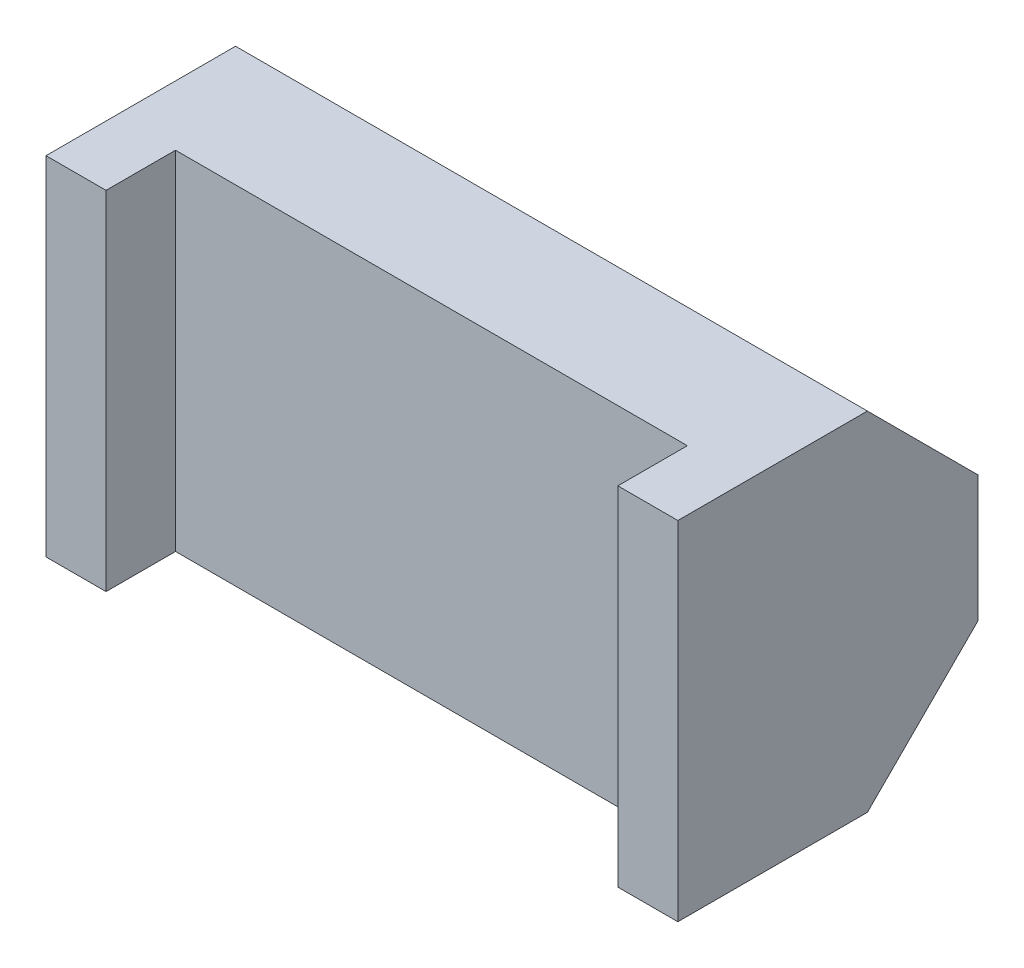
SolidWorks part; units mm, degrees
ref_plane "前视基准面" through (0, 0, 0) normal (0, 0, 1) x (1, 0, 0)
ref_plane "上视基准面" through (0, 0, 0) normal (0, 1, 0) x (1, 0, 0)
ref_plane "右视基准面" through (0, 0, 0) normal (1, 0, 0) x (0, 0, -1)
sketch "草图1" plane through (0, 0, 0) normal (0, 0, 1) x (1, 0, 0)
  line L0 (0, 5.5) -> (0, 0) construction
  line L1 (-10, 5.5) -> (10, 5.5)
  line L2 (-10, 5.5) -> (-10, -5.5)
  line L3 (-10, -5.5) -> (10, -5.5)
  line L4 (10, 5.5) -> (10, -5.5)
  line L5 (0, 0) -> (10, 0) construction
  dimension "D1" = 20
  dimension "D2" = 11
extrude "凸台-拉伸1" add sketch "草图1" along normal blind 9.5
sketch "草图2" plane through (0, 0, 9.5) normal (0, 0, 1) x (1, 0, 0)
  line L0 (0, 4.3603) -> (0, 0) construction
  line L1 (-8.1, 14.9476) -> (8.1, 14.9476)
  line L2 (-8.1, 14.9476) -> (-8.1, -14.9476)
  line L3 (-8.1, -14.9476) -> (8.1, -14.9476)
  line L4 (8.1, 14.9476) -> (8.1, -14.9476)
  line L5 (0, 0) -> (16.2, 0) construction
  dimension "D1" = 16.2
extrude "切除-拉伸1" cut sketch "草图2" against normal blind 2.2
sketch "草图3" plane through (-10, 0, 0) normal (-1, 0, 0) x (0, 0, 1)
  line L0 (0, 5.5) -> (3.5, 5.5)
  line L1 (9.5, 5.5) -> (0, 5.5) construction
  line L2 (3.5, 5.5) -> (0, 2)
  line L3 (0, 5.5) -> (0, -5.5) construction
  line L4 (0, 2) -> (0, 5.5)
  line L5 (0, 0) -> (3.2793, 0) construction
  dimension "D1" = 3.5
  dimension "D2" = 45
extrude "切除-拉伸2" cut sketch "草图3" against normal through all
mirror "镜向1" about plane through (0, 0, 0) normal (0, 1, 0) of "切除-拉伸2"
